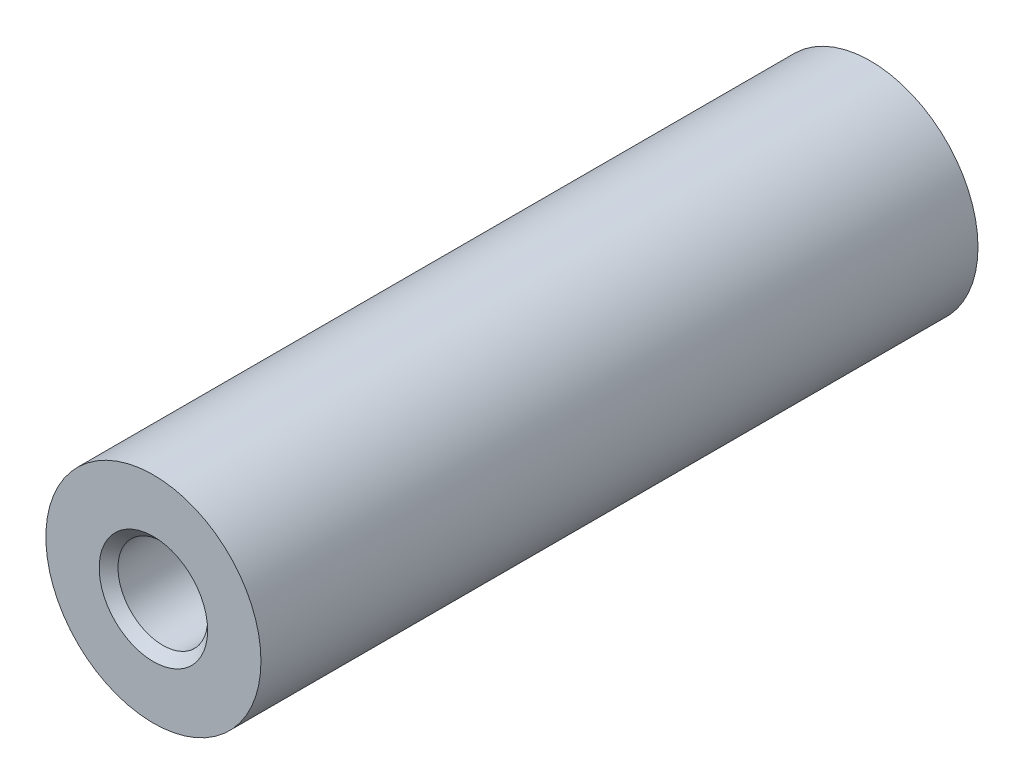
SolidWorks part; units mm, degrees
ref_plane "前视基准面" through (0, 0, 0) normal (0, 0, 1) x (1, 0, 0)
ref_plane "上视基准面" through (0, 0, 0) normal (0, 1, 0) x (1, 0, 0)
ref_plane "右视基准面" through (0, 0, 0) normal (1, 0, 0) x (0, 0, -1)
sketch "草图1" plane through (0, 0, 0) normal (0, 0, 1) x (1, 0, 0)
  circle A0 centre (0, 0) radius 6
  dimension "D1" = 12
extrude "凸台-拉伸1" add sketch "草图1" along normal mid plane 40
hole_wizard "M6 螺纹孔1" positions "3D草图1" profile "草图3" tap size "M6" standard "GB"
sketch3d "3D草图1"
  circle A0 centre (0, 0, 20) radius 6 construction
  point P0 (0, 0, 20)
  point P7 (0, 0, 26)
sketch "草图3" plane through (0, 0, 20) normal (1, 0, 0) x (0, -1, 0)
  line L0 (0, 0) -> (0, 10.5022)
  line L1 (0, 10.5022) -> (2.5, 9)
  line L2 (2.5, 9) -> (2.5, 0.525)
  line L3 (2.5, 0.525) -> (3.025, 0)
  line L5 (3.025, 0) -> (0, 0)
  line L6 (-2.5, 0.525) -> (-3.025, 0) construction
  line L10 (0, 10.5022) -> (-2.5, 9) construction
  line L11 (0, -6.35) -> (0, 107.95) construction
  dimension "螺纹孔钻头直径" = 5
  dimension "螺纹孔钻头深度" = 9
  dimension "近端锥形沉头孔直径" = 6.05
  dimension "近端锥形沉头孔角度" = 90
  dimension "导头角度" = 118
cosmetic thread "孔螺蚊线1" parameters "D1"=6, "D2"=6
mirror "镜向1" about plane through (0, 0, 0) normal (0, 0, 1) of "M6 螺纹孔1"
